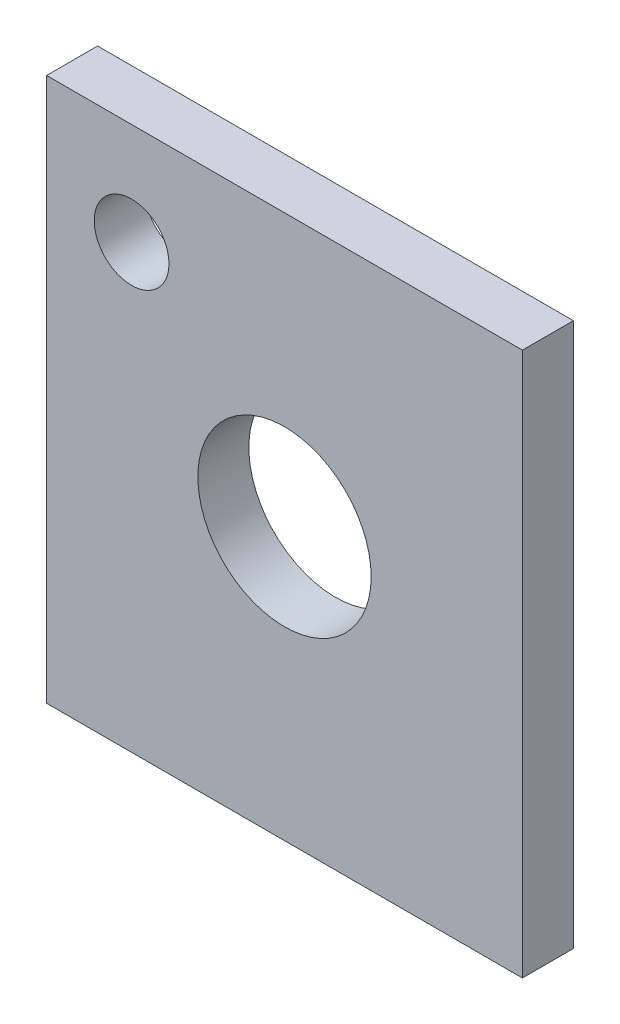
SolidWorks part; units mm, degrees
ref_plane "前视基准面" through (0, 0, 0) normal (0, 0, 1) x (1, 0, 0)
ref_plane "上视基准面" through (0, 0, 0) normal (0, 1, 0) x (1, 0, 0)
ref_plane "右视基准面" through (0, 0, 0) normal (1, 0, 0) x (0, 0, -1)
other "Configuration Table"
sketch "草图1" plane through (0, 0, 0) normal (0, 0, 1) x (1, 0, 0)
  line L0 (-14, -16) -> (14, -16)
  line L1 (14, -16) -> (14, 16)
  line L2 (14, 16) -> (-14, 16)
  line L3 (-14, 16) -> (-14, -16)
  point P0 (0, 0)
  dimension "D1" = 14
  dimension "D2" = 28
  dimension "D3" = 16
  dimension "D4" = 32
extrude "凸台-拉伸1" add sketch "草图1" against normal mid plane 3
sketch "草图2" plane through (0, 0, 0) normal (0, 0, 1) x (1, 0, 0)
  circle A0 centre (0, 0) radius 5.1
  circle A1 centre (-9, 10) radius 2.2
  point P0 (0, 0)
  dimension "D1" = 10.2
  dimension "D2" = 4.4
  dimension "D3" = 9
  dimension "D4" = 10
extrude "切除-拉伸1" cut sketch "草图2" against normal mid plane 23
